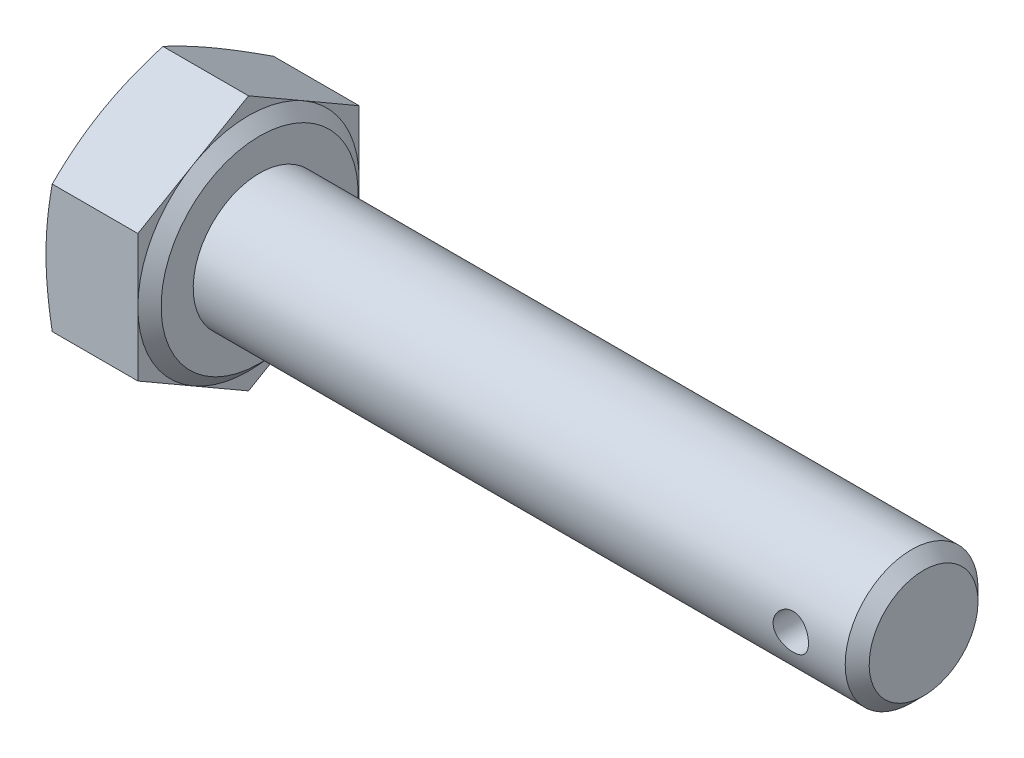
SolidWorks part; units mm, degrees
ref_plane "Front" through (0, 0, 0) normal (0, 0, 1) x (1, 0, 0)
ref_plane "Top" through (0, 0, 0) normal (0, 1, 0) x (1, 0, 0)
ref_plane "Right" through (0, 0, 0) normal (1, 0, 0) x (0, 0, -1)
other "Configuration Table"
sketch "Sketch-BaseHead" plane through (0, 0, 0) normal (1, 0, 0) x (0, 0, -1)
  line L1 (0, -5.7735) -> (5, -2.8868)
  line L2 (5, -2.8868) -> (5, 2.8868)
  line L3 (5, 2.8868) -> (0, 5.7735)
  line L4 (0, 5.7735) -> (-5, 2.8868)
  line L5 (-5, 2.8868) -> (-5, -2.8868)
  line L6 (-5, -2.8868) -> (0, -5.7735)
  circle A0 centre (0, 0) radius 5 construction
extrude "BaseHead" add sketch "Sketch-BaseHead" along normal blind 4.15
sketch "Sketch4" plane through (-0.2646, -5.9169, 0) normal (0, 0, 1) x (0, 1, 0)
  line L0 (5.9169, 3.7369) -> (5.9169, -10.4477) construction
  line L2 (11.6904, -0.2646) -> (10.9169, -0.2646)
  line L4 (10.9169, -0.2646) -> (11.6904, -0.5462)
  line L6 (11.6904, -0.5462) -> (11.6904, -0.2646)
revolve "HeadChamfer" cut sketch "Sketch4" angle 360 about L0
sketch "Sketch1" plane through (0, 0, 0) normal (0, 1, 0) x (1, 0, 0)
  line L0 (4.15, 0) -> (4.65, 0)
  line L1 (4.65, 0) -> (4.65, 4.45)
  line L2 (4.65, 4.45) -> (4.15, 5)
  line L3 (4.15, 5) -> (4.15, 0)
  line L6 (-4.0016, 0) -> (10.1831, 0) construction
revolve "Revolve1" add sketch "Sketch1" angle 360 about axis through (-4.0016, 0, 0) along (1, 0, 0)
ref_plane "Plane2" through (16.65, 0, 0) normal (1, 0, 0) x (0, 0, -1)
sketch "Sketch3" plane through (4.65, 0, 0) normal (1, 0, 0) x (0, 0, -1)
  circle A0 centre (0, 0) radius 3
extrude "BaseBody" add sketch "Sketch3" along normal blind 30
cosmetic thread "ThreadCosmetic1" [suppressed] parameters "b"=18, "D2"=4.917
chamfer "Chamfer1" distance 0.5415 angle 45 1 edges at (34.65, 3, 0)
fillet "HeadFillet" [suppressed] radius 0.25
sketch "Sketch5" plane through (0, 0, 0) normal (0, 0, 1) x (1, 0, 0)
  line L2 (4.65, -4.45) -> (4.65, 4.45) construction
  line L3 (34.1085, 0) -> (4.65, 0) construction
  circle A0 centre (31.65, 0) radius 0.8
  dimension "d1" = 1.6
  dimension "lh" = 27
extrude "Hole" cut sketch "Sketch5" against normal through all and the other way through all
sketch "Sketch6" plane through (0, 0, 0) normal (0, 0, 1) x (1, 0, 0)
  line L0 (33.566, 3.2) -> (34.1075, 3.2)
  line L1 (34.1075, 3.2) -> (34.1075, 3)
  line L2 (34.1075, 3) -> (33.8367, 2.531)
  line L3 (33.566, 3) -> (33.8367, 2.531)
  line L4 (33.566, 3.2) -> (33.566, 3)
  line L5 (27.8988, 0) -> (0, 0) construction
  line L6 (33.566, 3) -> (34.1075, 3) construction
  line L7 (33.8367, 3) -> (33.8367, 2.531) construction
  line L8 (34.1085, 3) -> (4.65, 3) construction
  point P5 (33.8367, 3.2)
revolve "Cut-Revolve10" [suppressed] cut sketch "Sketch6" angle 360 about L5
pattern_linear "LPattern10" [suppressed] count 28 spacing 0.6498
equation "\"D1@Sketch1\" = \"s@Sketch-BaseHead\" / 2"
equation "\"D2@Sketch4\" = \"s@Sketch-BaseHead\""
equation "\"D1@Chamfer1\" = (  \"d@Sketch3\"  -\"D2@ThreadCosmetic1\" ) / 2 "
equation "\"b@ThreadCosmetic1\" = \"l@BaseBody\" - \"lg@Plane2\""
equation "\"D2@Sketch6\" = (  \"d@Sketch3\" - \"D2@ThreadCosmetic1\" )  / 2"
equation "\"D3@LPattern10\" =\"D2@Sketch6\" * 1.2"
equation "\"D1@LPattern10\" = \"b@ThreadCosmetic1\" / \"D3@LPattern10\""
equation "\"D3@Sketch6\" = 0.001"
